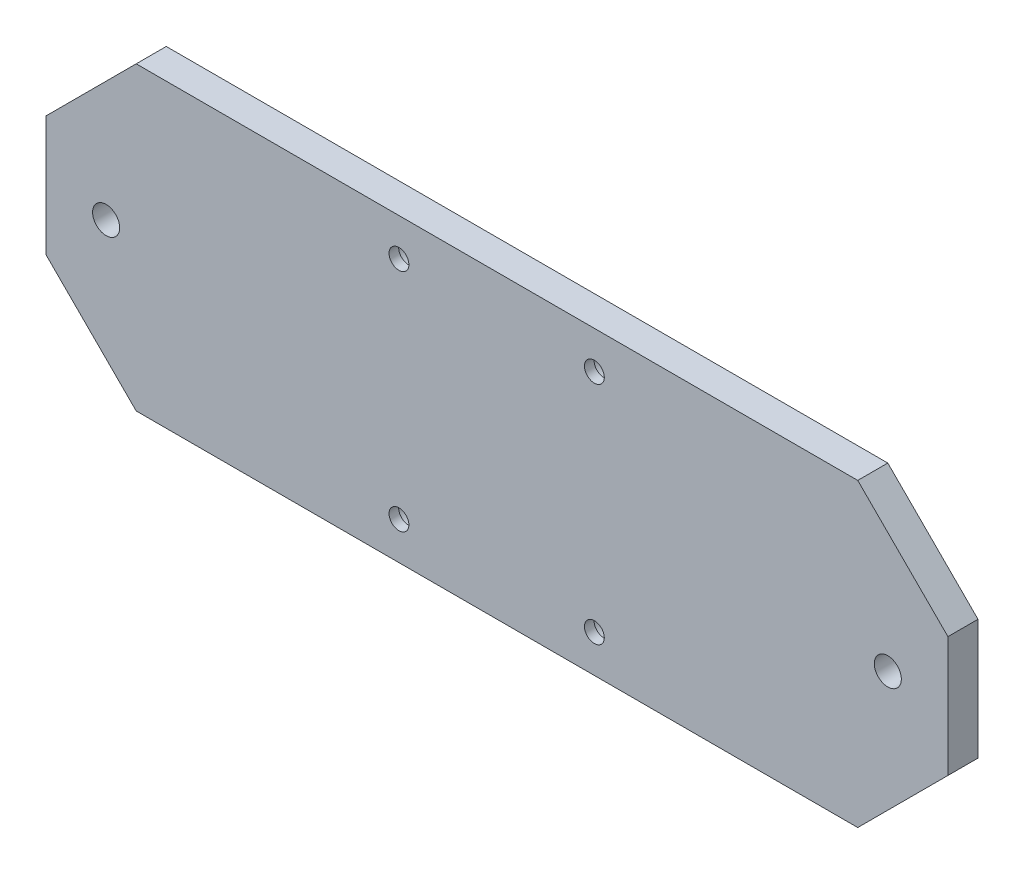
from build123d import *

# Parameters (mm, degrees)
SKETCH_1_W                = 300
SKETCH_1_H                = 100
EXTRUDE_1_DEPTH           = 10
HOLE_WIZARD_1_D           = 6.6
HOLE_WIZARD_1_CBORE_D     = 11
HOLE_WIZARD_1_CBORE_DEPTH = 6.8
HOLE_WIZARD_M8_1_D        = 9
CHAMFER_1_SIZE            = 30


with BuildPart() as part:
    # 草图1 → 凸台-拉伸1 (new body)
    with BuildSketch(Plane.XY):
        Rectangle(SKETCH_1_W, SKETCH_1_H)
    extrude(amount=EXTRUDE_1_DEPTH)

    # 打孔尺寸(%根据)内六角圆柱头螺钉的类型1 (through all)
    with Locations(Plane(origin=(0, 0, 0), x_dir=(-1, 0, 0), z_dir=(0, 0, -1))):
        with Locations((32.599999971, -37.5), (-32.400000029, -37.5), (-32.400000029, 37.5), (32.599999971, 37.5)):
            CounterBoreHole(HOLE_WIZARD_1_D / 2, HOLE_WIZARD_1_CBORE_D / 2, HOLE_WIZARD_1_CBORE_DEPTH)

    # M8 间隙孔1 (through all)
    with Locations(Plane(origin=(0, 0, 0), x_dir=(-1, 0, 0), z_dir=(0, 0, -1))):
        with Locations((-130, 0), (130, 0)):
            Hole(HOLE_WIZARD_M8_1_D / 2)

    # 倒角1
    chamfer_1_edges = [part.edges().sort_by_distance(p)[0] for p in [
        (-150, 50, 5),
        (150, 50, 5),
        (150, -50, 5),
        (-150, -50, 5),
    ]]
    chamfer(chamfer_1_edges, length=CHAMFER_1_SIZE)


solid = part.part
